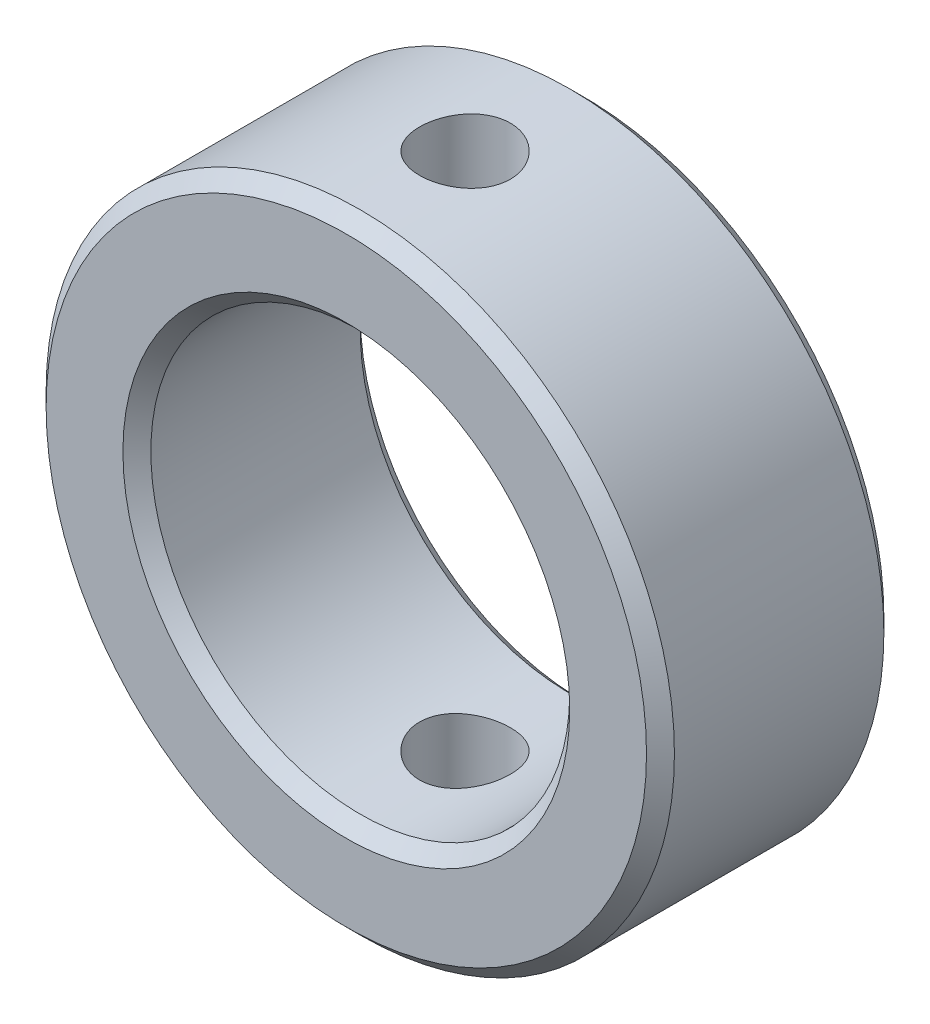
SolidWorks part; units mm, degrees
ref_plane "Front Plane" through (0, 0, 0) normal (0, 0, 1) x (1, 0, 0)
ref_plane "Top Plane" through (0, 0, 0) normal (0, 1, 0) x (1, 0, 0)
ref_plane "Right Plane" through (0, 0, 0) normal (1, 0, 0) x (0, 0, -1)
sketch "Sketch1" plane through (0, 0, 0) normal (0, 0, 1) x (1, 0, 0)
  circle A0 centre (0, 0) radius 30
  circle A1 centre (0, 0) radius 45
  dimension "D1" = 60
  dimension "D2" = 90
extrude "Boss-Extrude1" add sketch "Sketch1" along normal blind 34
sketch "Sketch2" plane through (0, 0, 0) normal (0, 1, 0) x (1, 0, 0)
  line L0 (0, 0) -> (0, -60.2523) construction
  circle A0 centre (0, -17) radius 6.5
  dimension "D2" = 13
  dimension "D1" = 17
extrude "Cut-Extrude1" cut sketch "Sketch2" against normal through all and the other way through all
chamfer "Chamfer1" distance 2 angle 45 4 edges at (30, 0, 0) (45, 0, 0) (30, 0, 34) (45, 0, 34)
